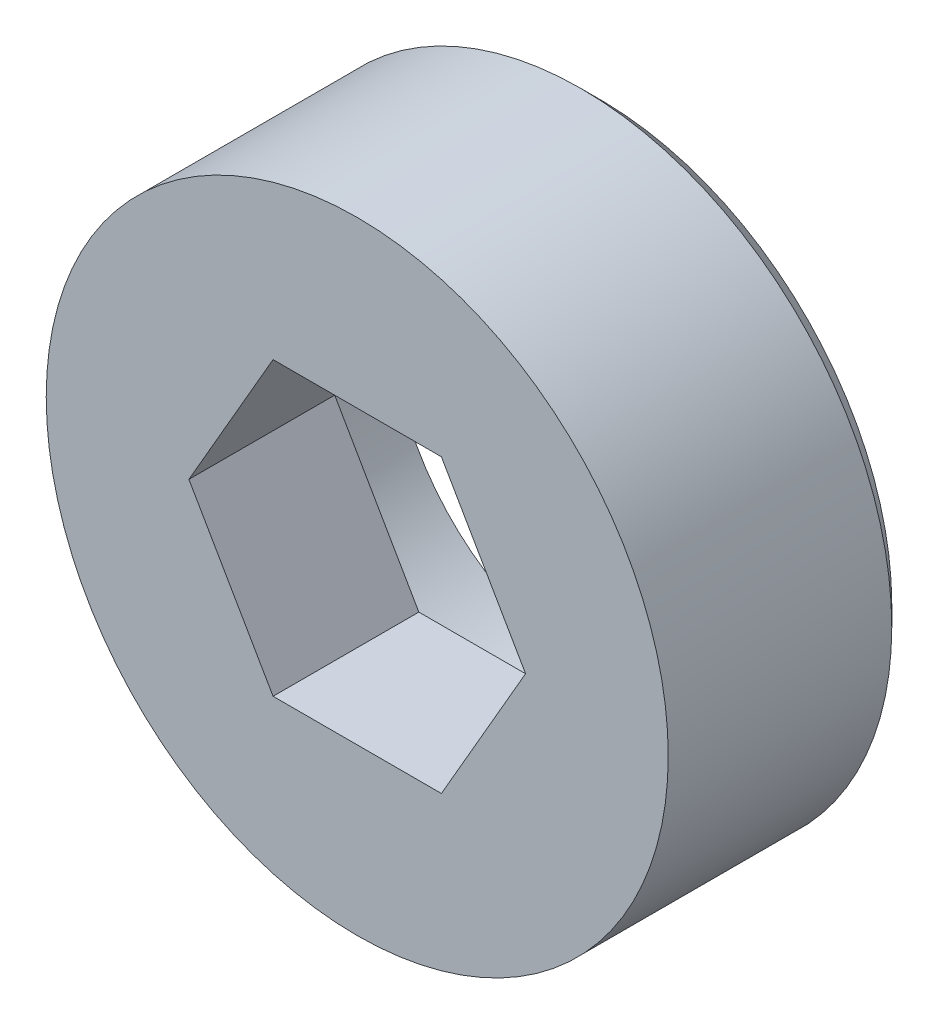
from build123d import *

# Parameters (mm, degrees)
SKETCH_1_R          = 32
EXTRUDE_1_DEPTH     = 25
CUT_EXTRUDE_1_DEPTH = 52.701063819
SKETCH_3_R          = 21.5
CUT_EXTRUDE_2_DEPTH = 10
CHAMFER_1_SIZE      = 2


with BuildPart() as part:
    # 草图1 → 凸台-拉伸1 (new body)
    with BuildSketch(Plane.XY):
        Circle(SKETCH_1_R)
    extrude(amount=EXTRUDE_1_DEPTH)

    # 草图2 → 切除-拉伸1 (cut, through all)
    with BuildSketch(Plane.XY.offset(25)):
        Polygon((17.320508076, 0), (8.660254038, 15), (-8.660254038, 15), (-17.320508076, 0), (-8.660254038, -15), (8.660254038, -15), align=None)
    extrude(amount=-CUT_EXTRUDE_1_DEPTH, mode=Mode.SUBTRACT)

    # 草图3 → 切除-拉伸2 (cut)
    with BuildSketch(Plane(origin=(0, 0, 0), x_dir=(-1, 0, 0), z_dir=(0, 0, -1))):
        Circle(SKETCH_3_R)
    extrude(amount=-CUT_EXTRUDE_2_DEPTH, mode=Mode.SUBTRACT)

    # 倒角1
    chamfer_1_edges = [part.edges().sort_by_distance(p)[0] for p in [
        (-32, 0, 0),
    ]]
    chamfer(chamfer_1_edges, length=CHAMFER_1_SIZE)


solid = part.part
